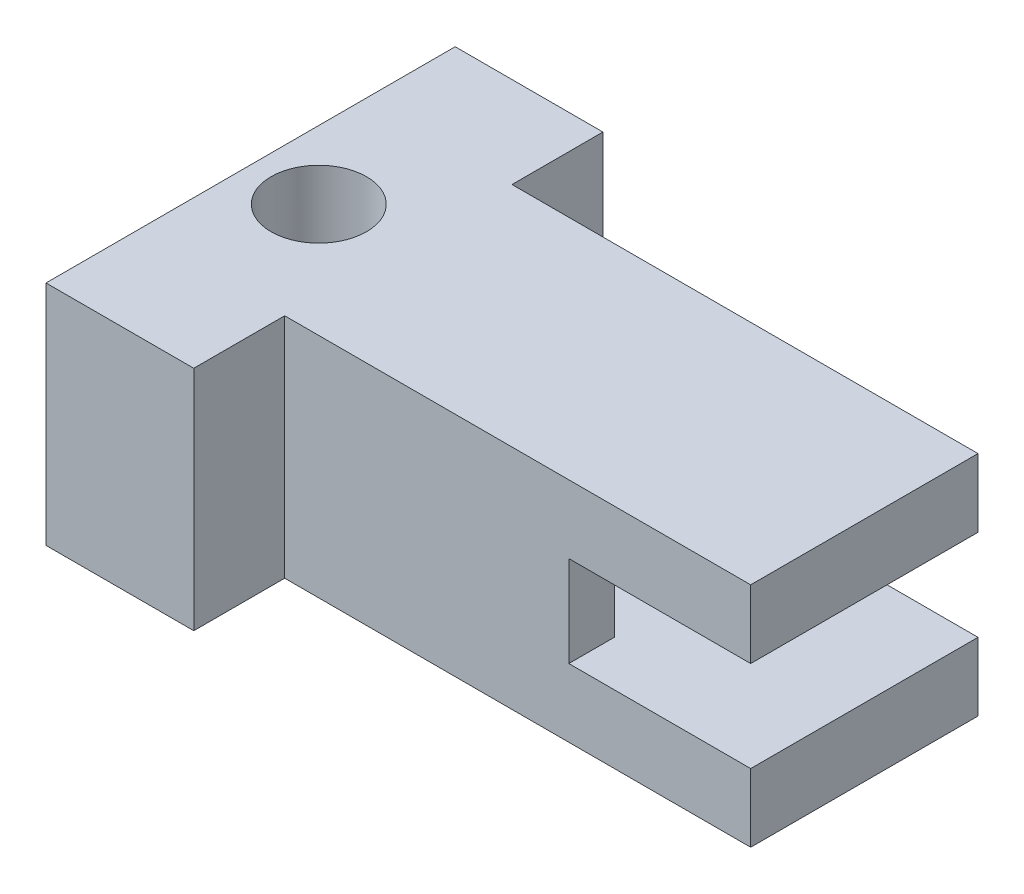
from build123d import *

# Parameters (mm, degrees)
SKETCH1_W                   = 16
SKETCH1_H                   = 10
BOSS_EXTRUDE1_DEPTH         = 10
SKETCH2_W                   = 16
SKETCH2_H                   = 4
CUT_EXTRUDE1_DEPTH          = 10
SKETCH3_W                   = 10
SKETCH3_H                   = 10
BOSS_EXTRUDE2_DEPTH         = 7
SKETCH4_W                   = 2.5
SKETCH4_H                   = 10
BOSS_EXTRUDE3_DEPTH         = 4
SKETCH5_W                   = 6
SKETCH5_H                   = 4
CUT_EXTRUDE2_DEPTH          = 4
SKETCH6_R                   = 1
BOSS_EXTRUDE4_DEPTH         = 3
SKETCH7_R                   = 1.3
BOSS_EXTRUDE5_DEPTH         = 1
SKETCH8_W                   = 18
SKETCH8_H                   = 10
BOSS_EXTRUDE6_DEPTH         = 4
TAP_DRILL_FOR_M5_TAP1_D     = 4.2
TAP_DRILL_FOR_M5_TAP1_DEPTH = 60
TAP_DRILL_FOR_M5_TAP1_TIP   = 1.2618073


with BuildPart() as part:
    # Sketch1 → Boss-Extrude1 (new body)
    with BuildSketch(Plane(origin=(0, 0, 0), x_dir=(1, 0, 0), z_dir=(0, 1, 0))):
        Rectangle(SKETCH1_W, SKETCH1_H)
    extrude(amount=BOSS_EXTRUDE1_DEPTH)

    # Sketch2 → Cut-Extrude1 (cut)
    with BuildSketch(Plane(origin=(0, 0, -5), x_dir=(-1, 0, 0), z_dir=(0, 0, -1))):
        with Locations((-8, 5)):
            Rectangle(SKETCH2_W, SKETCH2_H)
    extrude(amount=-CUT_EXTRUDE1_DEPTH, mode=Mode.SUBTRACT)

    # Sketch3 → Boss-Extrude2 (add)
    with BuildSketch(Plane.ZY.offset(8)):
        with Locations((0, 5)):
            Rectangle(SKETCH3_W, SKETCH3_H)
    extrude(amount=BOSS_EXTRUDE2_DEPTH)

    # Sketch4 → Boss-Extrude3 (add)
    with BuildSketch(Plane(origin=(0, 0, -5), x_dir=(-1, 0, 0), z_dir=(0, 0, -1))):
        with Locations((13.75, 5)):
            Rectangle(SKETCH4_W, SKETCH4_H)
    boss_extrude3 = extrude(amount=BOSS_EXTRUDE3_DEPTH)

    # Mirror1: Boss-Extrude3 across plane
    add(boss_extrude3.mirror(Plane(origin=(0, 0, 0), x_dir=(1, 0, 0), z_dir=(0, 0, -1))))

    # Sketch5 → Cut-Extrude2 (cut)
    with BuildSketch(Plane(origin=(0, 0, 0), x_dir=(0, 0, -1), z_dir=(1, 0, 0))):
        with Locations((0, 5)):
            Rectangle(SKETCH5_W, SKETCH5_H)
    extrude(amount=-CUT_EXTRUDE2_DEPTH, mode=Mode.SUBTRACT)

    # Sketch6 → Boss-Extrude4 (add)
    with BuildSketch(Plane(origin=(-4, 0, 0), x_dir=(0, 0, -1), z_dir=(1, 0, 0))):
        with Locations((0, 5)):
            Circle(SKETCH6_R)
    extrude(amount=BOSS_EXTRUDE4_DEPTH)

    # Sketch7 → Boss-Extrude5 (add)
    with BuildSketch(Plane(origin=(-1, 0, 0), x_dir=(0, 0, -1), z_dir=(1, 0, 0))):
        with Locations((0, 5)):
            Circle(SKETCH7_R)
    extrude(amount=-BOSS_EXTRUDE5_DEPTH)

    # Sketch8 → Boss-Extrude6 (add)
    with BuildSketch(Plane.ZY.offset(15)):
        with Locations((0, 5)):
            Rectangle(SKETCH8_W, SKETCH8_H)
    extrude(amount=BOSS_EXTRUDE6_DEPTH)

    # Tap Drill for M5 Tap1
    with Locations(Plane.XZ):
        with Locations((-16, 0)):
            Hole(TAP_DRILL_FOR_M5_TAP1_D / 2, depth=TAP_DRILL_FOR_M5_TAP1_DEPTH)
            with Locations((0, 0, -(TAP_DRILL_FOR_M5_TAP1_DEPTH + TAP_DRILL_FOR_M5_TAP1_TIP / 2))):  # 118° drill point
                Cone(0, TAP_DRILL_FOR_M5_TAP1_D / 2, TAP_DRILL_FOR_M5_TAP1_TIP, mode=Mode.SUBTRACT)


solid = part.part
